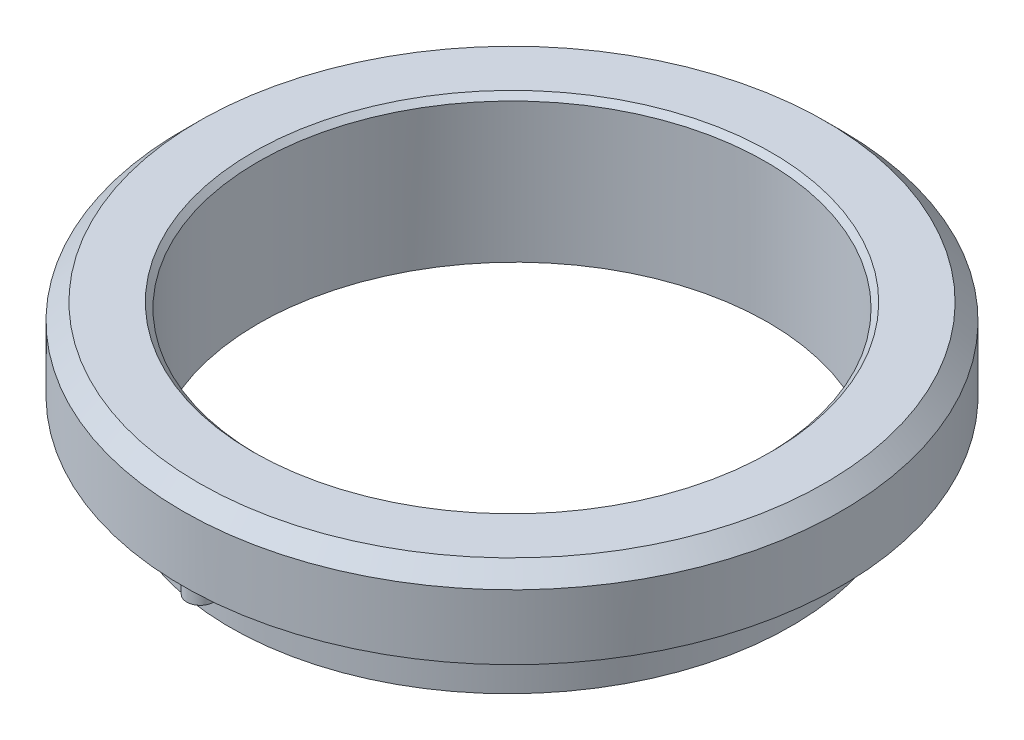
from build123d import *

# Parameters (mm, degrees)
CUT_EXTRUDE_1_DEPTH      = 44.780703512
CUT_EXTRUDE_1_DEPTH_BACK = 44.780703512
CHAMFER_1_SIZE           = 0.5
CHAMFER_2_SIZE           = 1.5
SKETCH_3_R               = 1.25
EXTRUDE_1_DEPTH          = 1.5


with BuildPart() as part:
    # 草图1 → 旋转1 (revolve)
    with BuildSketch(Plane.XY, mode=Mode.PRIVATE) as revolve_1_sk:
        Polygon((23.5, -7.5), (23.5, 7.5), (30.5, 7.5), (30.5, 0), (27.35, 0), (27.35, 1), (25.85, 1), (25.85, -7.5), align=None)
    revolve(revolve_1_sk.sketch.rotate(Axis((0, 0, 0), (0, 1, 0)), 90), axis=Axis((0, 0, 0), (0, 1, 0)))

    # 草图2 → 切除-拉伸1 (cut, two sides: drawn at the far end of the back side and taken through both)
    with BuildSketch(Plane.XY.offset(-CUT_EXTRUDE_1_DEPTH_BACK)):
        Polygon((-25.85, -6), (25.85, -5.548820935), (25.85, -7.5), (-25.85, -7.5), align=None)
    extrude(amount=CUT_EXTRUDE_1_DEPTH + CUT_EXTRUDE_1_DEPTH_BACK, mode=Mode.SUBTRACT)

    # 倒角1
    chamfer_1_edges = [part.edges().sort_by_distance(p)[0] for p in [
        (0, 7.5, 23.5),
    ]]
    chamfer(chamfer_1_edges, length=CHAMFER_1_SIZE)

    # 倒角2
    chamfer_2_edges = [part.edges().sort_by_distance(p)[0] for p in [
        (0, 7.5, 30.5),
    ]]
    chamfer(chamfer_2_edges, length=CHAMFER_2_SIZE)

    # 草图3 → 凸台-拉伸1 (add)
    with BuildSketch(Plane.XZ):
        with Locations(Location((0, 28.85, 0), (0, 0, 270))):
            Circle(SKETCH_3_R)
    extrude(amount=EXTRUDE_1_DEPTH)


solid = part.part
